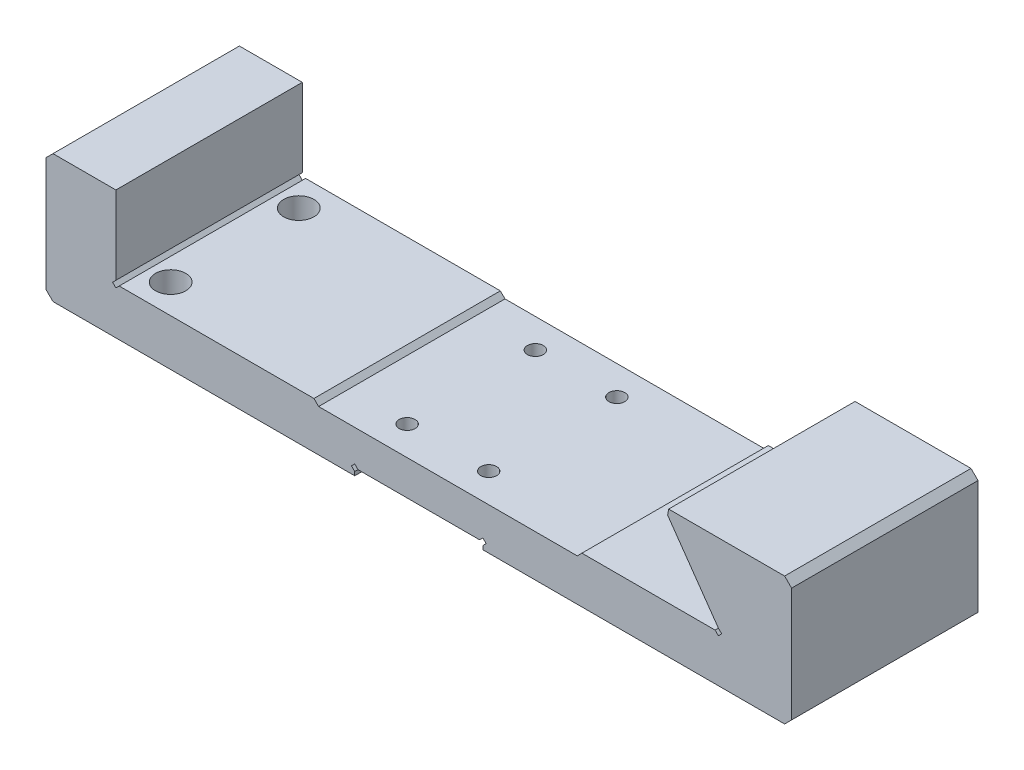
SolidWorks part; units mm, degrees
ref_plane "Front Plane" through (0, 0, 0) normal (0, 0, 1) x (1, 0, 0)
ref_plane "Top Plane" through (0, 0, 0) normal (0, 1, 0) x (1, 0, 0)
ref_plane "Right Plane" through (0, 0, 0) normal (1, 0, 0) x (0, 0, -1)
other "Configuration Table"
sketch "Sketch1" plane through (0, 0, 0) normal (0, 1, 0) x (1, 0, 0)
  line L1 (-160, -40) -> (160, -40)
  line L2 (-160, -40) -> (-160, 40)
  line L3 (-160, 40) -> (160, 40)
  line L4 (160, -40) -> (160, 40)
  line L5 (-160, -40) -> (160, 40) construction
  line L6 (-160, 40) -> (160, -40) construction
  point P0 (0, 0)
  dimension "D1" = 320
  dimension "D2" = 80
extrude "Boss-Extrude1" add sketch "Sketch1" along normal blind 55
sketch "Sketch2" plane through (0, 0, 40) normal (0, 0, 1) x (1, 0, 0)
  line L0 (105.0688, 55) -> (128.5858, 21.4142)
  line L1 (-160, 55) -> (160, 55) construction
  line L3 (-130, 21.4142) -> (-130, 55)
  line L4 (-130, 55) -> (105.0688, 55)
  line L5 (-130, 21.4142) -> (-131.4142, 20)
  line L6 (-131.4142, 20) -> (-130, 18.5858)
  line L7 (-130, 18.5858) -> (-128.5858, 20)
  line L8 (-128.5858, 20) -> (-45, 20)
  line L9 (-45, 20) -> (-43, 18)
  line L10 (-43, 18) -> (68, 18)
  line L11 (68, 18) -> (70, 20)
  line L12 (70, 20) -> (127.1716, 20)
  line L13 (127.1716, 20) -> (128.5858, 18.5858)
  line L14 (128.5858, 18.5858) -> (130, 20)
  line L15 (130, 20) -> (128.5858, 21.4142)
  line L17 (-160, 0) -> (160, 0) construction
  line L19 (-160, 55) -> (-160, 0) construction
  line L21 (130, 20) -> (130, 55) construction
  dimension "D1" = 2
  dimension "D2" = 2
  dimension "D3" = 60
  dimension "D4" = 135
  dimension "D5" = 85
  dimension "D6" = 2
  dimension "D7" = 2
  dimension "D8" = 260
  dimension "D9" = 55
  dimension "D10" = 45
  dimension "D11" = 60
  dimension "D12" = 2
  dimension "D13" = 35
  dimension "D14" = 2
  dimension "D15" = 2
  dimension "D16" = 2
  dimension "D17" = 30
extrude "Cut-Extrude1" cut sketch "Sketch2" against normal through all
sketch "Sketch3" plane through (0, 0, 40) normal (0, 0, 1) x (1, 0, 0)
  line L0 (0, 0) -> (0, 3) construction
  line L1 (-26.0858, 3) -> (26.0858, 3)
  line L2 (26.0858, 3) -> (27.5, 4.4142)
  line L3 (27.5, 4.4142) -> (28.9142, 3)
  line L4 (28.9142, 3) -> (27.5, 1.5858)
  line L5 (27.5, 1.5858) -> (27.5, 0)
  line L6 (-160, 0) -> (160, 0) construction
  line L7 (27.5, 0) -> (-27.5, 0)
  line L8 (-43, 18) -> (68, 18) construction
  line L9 (-27.5, 1.5858) -> (-27.5, 0)
  line L10 (-28.9142, 3) -> (-27.5, 1.5858)
  line L11 (-27.5, 4.4142) -> (-28.9142, 3)
  line L12 (-26.0858, 3) -> (-27.5, 4.4142)
  dimension "D1" = 27.5
  dimension "D2" = 2
  dimension "D3" = 45
  dimension "D4" = 2
  dimension "D5" = 15
  dimension "D6" = 2
extrude "Cut-Extrude2" cut sketch "Sketch3" against normal through all
sketch "Sketch4" plane through (0, 3, 0) normal (0, -1, 0) x (1, 0, 0)
  line L0 (0, 0) -> (0, -27.5) construction
  line L1 (0, -27.5) -> (17.5, -27.5) construction
  dimension "D1" = 35
  dimension "D2" = 27.5
hole_wizard "M8 Tapped Hole1" positions "Sketch5" profile "Sketch6" tap size "M8" standard "GB"
sketch "Sketch5" plane through (0, 3, 0) normal (0, -1, 0) x (-1, 0, 0)
  point P0 (-17.5, 27.5)
sketch "Sketch6" plane through (17.5, 3, -27.5) normal (1, 0, 0) x (0, 0, -1)
  line L0 (0, 0) -> (0, 21.7929)
  line L1 (0, 21.7929) -> (3.4, 19.75)
  line L2 (3.4, 19.75) -> (3.4, 0.625)
  line L3 (3.4, 0.625) -> (4.025, 0)
  line L5 (4.025, 0) -> (0, 0)
  line L6 (-3.4, 0.625) -> (-4.025, 0) construction
  line L10 (0, 21.7929) -> (-3.4, 19.75) construction
  line L11 (0, -6.35) -> (0, 107.95) construction
  dimension "螺纹孔钻头直径" = 6.8
  dimension "螺纹孔钻头深度" = 19.75
  dimension "近端锥形沉头孔直径" = 8.05
  dimension "近端锥形沉头孔角度" = 90
  dimension "导头角度" = 118
cosmetic thread "Hole Thread1" parameters "D1"=16, "D2"=8
mirror "Mirror1" about plane through (0, 0, 0) normal (1, 0, 0) of "M8 Tapped Hole1"
mirror "Mirror2" about plane through (0, 0, 0) normal (0, 0, 1) of "Mirror1", "M8 Tapped Hole1"
sketch "Sketch7" plane through (0, 20, 0) normal (0, 1, 0) x (1, 0, 0)
  line L0 (-130, 40) -> (-130, -40) construction
  line L1 (0, 0) -> (21.1838, 0) construction
  circle A0 centre (-119, 27.5) radius 6.5
  circle A1 centre (-119, -27.5) radius 6.5
  dimension "D2" = 13
  dimension "D1" = 11
  dimension "D3" = 27.5
extrude "Cut-Extrude3" cut sketch "Sketch7" against normal through all
chamfer "Chamfer1" distance 3 angle 45 5 edges at (160, 0, 0) (160, 55, 0) (105.0688, 55, 0) (-160, 0, 0) (-160, 55, 0)
